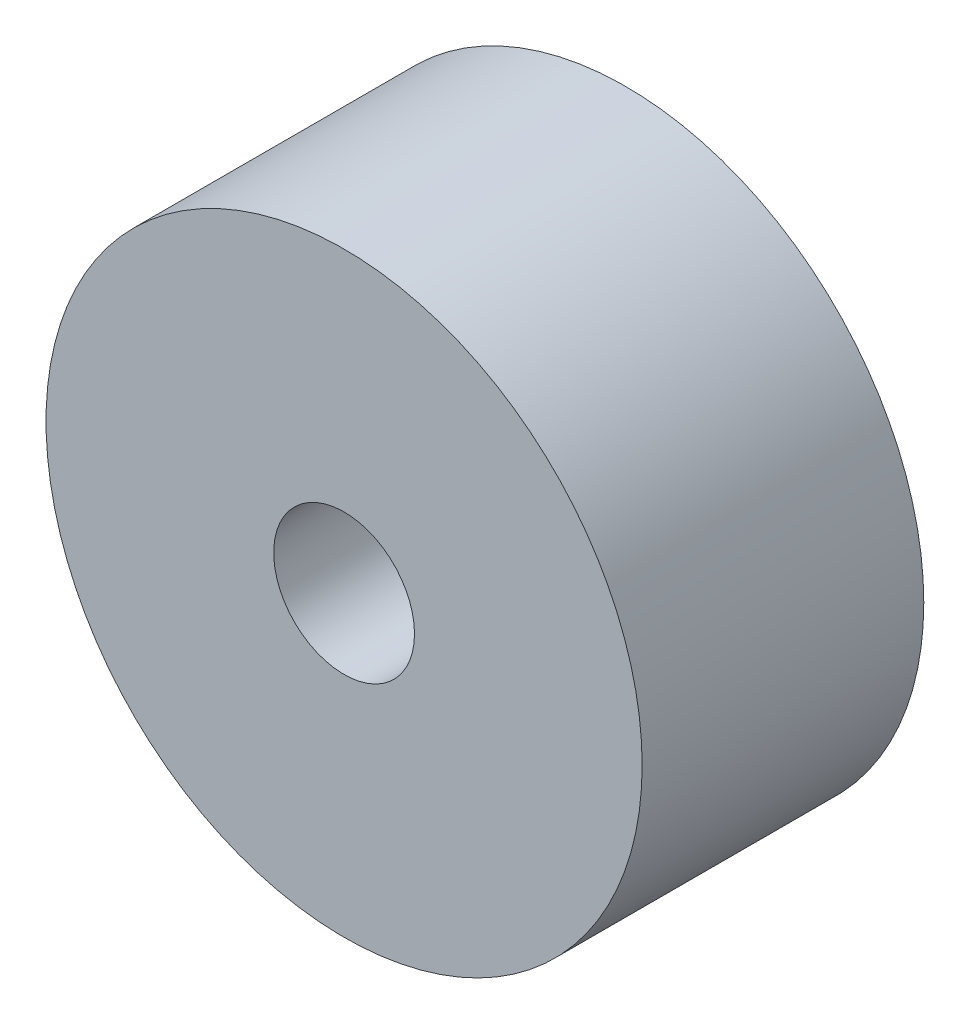
SolidWorks part; units mm, degrees
ref_plane "Front Plane" through (0, 0, 0) normal (0, 0, 1) x (1, 0, 0)
ref_plane "Top Plane" through (0, 0, 0) normal (0, 1, 0) x (1, 0, 0)
ref_plane "Right Plane" through (0, 0, 0) normal (1, 0, 0) x (0, 0, -1)
other "Configuration Table"
sketch "Sketch1" plane through (0, 0, 0) normal (0, 0, 1) x (1, 0, 0)
  circle A0 centre (0, 0) radius 12.7
  circle A1 centre (0, 0) radius 3
  dimension "D1" = 25.4
  dimension "D2" = 6
extrude "Boss-Extrude1" add sketch "Sketch1" along normal blind 12
